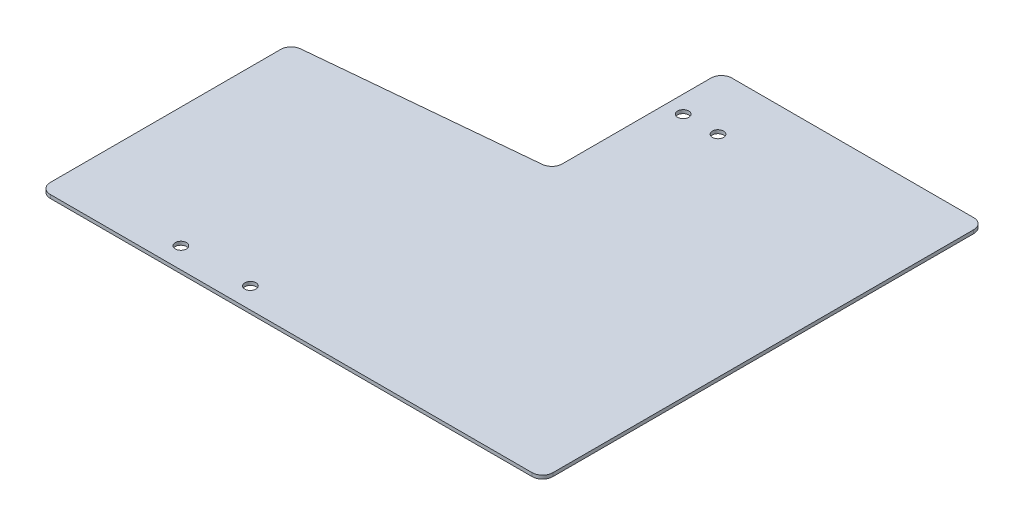
SolidWorks part; units mm, degrees
material "哈碳纤"
ref_plane "前视基准面" through (0, 0, 0) normal (0, 0, 1) x (1, 0, 0)
ref_plane "上视基准面" through (0, 0, 0) normal (0, 1, 0) x (1, 0, 0)
ref_plane "右视基准面" through (0, 0, 0) normal (1, 0, 0) x (0, 0, -1)
other "Configuration Table"
sketch "草图1" plane through (0, 0, 0) normal (0, 1, 0) x (1, 0, 0)
  line L0 (0, 0) -> (0, 72)
  line L1 (0, 72) -> (69, 78.5)
  line L2 (69, 78.5) -> (69, 127)
  line L3 (69, 127) -> (144.55, 127)
  line L4 (144.55, 127) -> (144.55, 0)
  line L5 (144.55, 0) -> (0, 0)
  circle A0 centre (74, 111) radius 1.6
  circle A1 centre (84, 111) radius 1.6
  circle A2 centre (34.55, 6) radius 1.6
  circle A3 centre (54.55, 6) radius 1.6
  point P15 (0, 0)
  dimension "D6" = 10
  dimension "D8" = 3.2
  dimension "D10" = 20
  dimension "D1" = 144.55
  dimension "D2" = 127
  dimension "D3" = 75.55
  dimension "D4" = 48.5
  dimension "D5" = 72
  dimension "D7" = 5
  dimension "D9" = 16
  dimension "D11" = 6
  dimension "D12" = 90
extrude "凸台-拉伸1" add sketch "草图1" along normal blind 1
fillet "圆角1" radius 3 6 edges at (0, 0.5, 0) (0, 0.5, -72) (69, 0.5, -78.5) (69, 0.5, -127) (144.55, 0.5, -127) (144.55, 0.5, 0)
